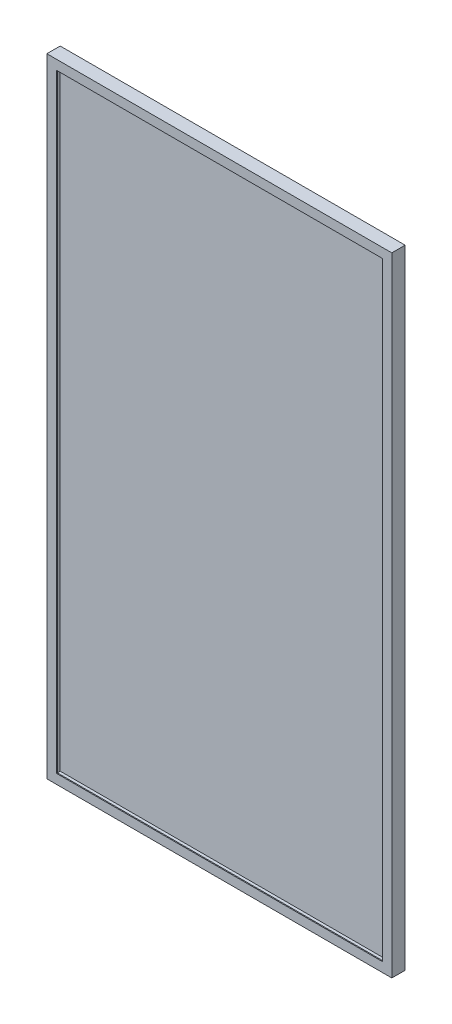
from build123d import *

# Parameters (mm, degrees)
SKETCH_1_W      = 724.5
SKETCH_1_H      = 1319
EXTRUDE_1_DEPTH = 28
SHELL_1_T       = -2
SKETCH_2_W      = 724.5
SKETCH_2_H      = 1319
SKETCH_2_W_2    = 684.5
SKETCH_2_H_2    = 1279
EXTRUDE_2_DEPTH = 2


with BuildPart() as part:
    # 草图1 → 凸台-拉伸1 (new body)
    with BuildSketch(Plane.XY):
        with Locations((362.25, 659.5)):
            Rectangle(SKETCH_1_W, SKETCH_1_H)
    extrude(amount=EXTRUDE_1_DEPTH)

    # 抽壳1
    shell_1_openings = [part.faces().sort_by_distance(p)[0] for p in [
        (362.25, 659.5, 28),
    ]]
    offset(amount=SHELL_1_T, openings=shell_1_openings, kind=Kind.INTERSECTION)

    # 草图2 → 凸台-拉伸2 (add)
    with BuildSketch(Plane.XY.offset(28)):
        with Locations((362.25, 659.5)):
            Rectangle(SKETCH_2_W, SKETCH_2_H)
        with Locations((362.25, 659.5)):
            Rectangle(SKETCH_2_W_2, SKETCH_2_H_2, mode=Mode.SUBTRACT)
    extrude(amount=-EXTRUDE_2_DEPTH)


solid = part.part
